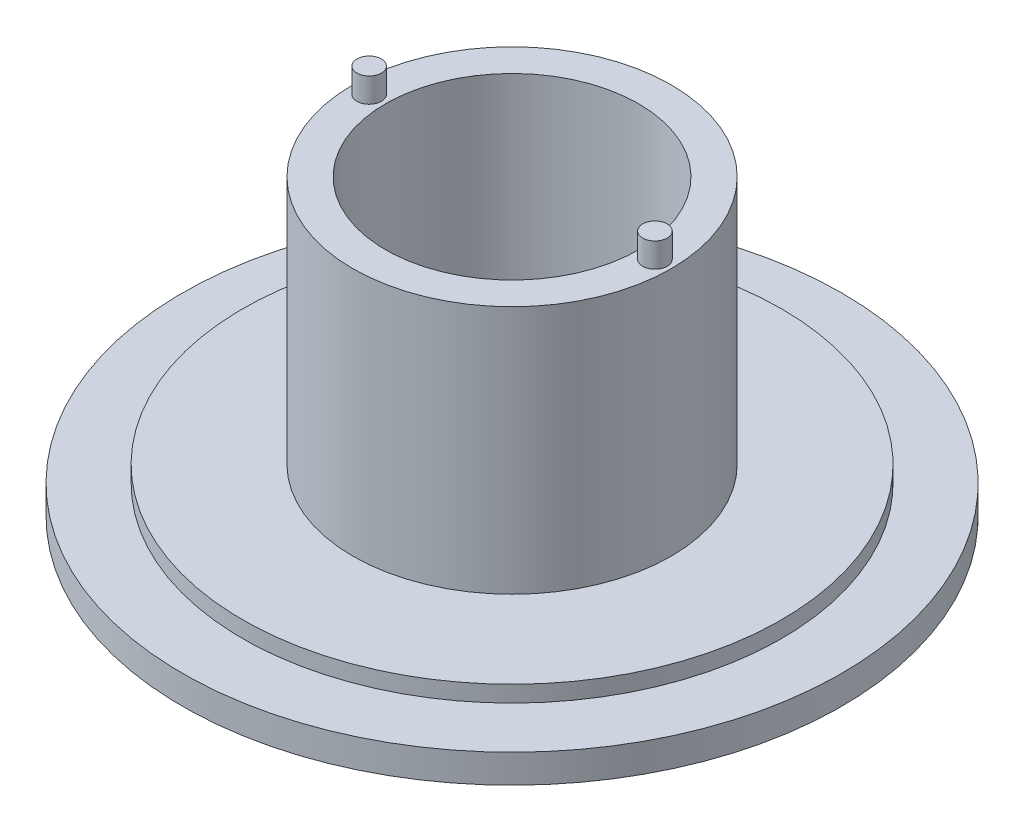
SolidWorks part; units mm, degrees
ref_plane "Front Plane" through (0, 0, 0) normal (0, 0, 1) x (1, 0, 0)
ref_plane "Top Plane" through (0, 0, 0) normal (0, 1, 0) x (1, 0, 0)
ref_plane "Right Plane" through (0, 0, 0) normal (1, 0, 0) x (0, 0, -1)
sketch "Sketch1" plane through (0, 0, 0) normal (0, 0, 1) x (1, 0, 0)
  line L0 (40.3687, 141) -> (33, 141)
  line L1 (-41, 141) -> (41, 141) construction
  line L2 (-33, 141) -> (33, 141) construction
  line L3 (33, 141) -> (33, 143)
  line L4 (33, 143) -> (-33, 143) construction
  line L5 (51, 143) -> (-51, 143) construction
  line L6 (33, 143) -> (19.5, 143)
  line L8 (19.5, 143) -> (19.5, 173.5)
  line L9 (20.2841, 173.5) -> (-20.2841, 173.5) construction
  line L10 (-60.9957, 137.5) -> (60.9957, 137.5) construction
  line L11 (29.3043, 137.5) -> (40.3687, 137.5)
  line L12 (40.3687, 137.5) -> (40.3687, 141)
  line L13 (19.5, 173.5) -> (15.5, 173.5)
  line L14 (15.5, 173.5) -> (15.5, 137.5)
  line L15 (15.5, 137.5) -> (29.3043, 137.5)
  line L16 (0, 0) -> (0, 33.1148) construction
revolve "Revolve1" add sketch "Sketch1" angle 360 about L16
sketch "Sketch2" plane through (0, 173.5, 0) normal (0, 1, 0) x (1, 0, 0)
  circle A0 centre (17.5, 0) radius 1.5
  circle A1 centre (-17.5, 0) radius 1.5
  circle A2 centre (0, 0) radius 15.5 construction
  dimension "D1" = 17.5
  dimension "D2" = 17.5
extrude "Boss-Extrude1" add sketch "Sketch2" along normal blind 3
